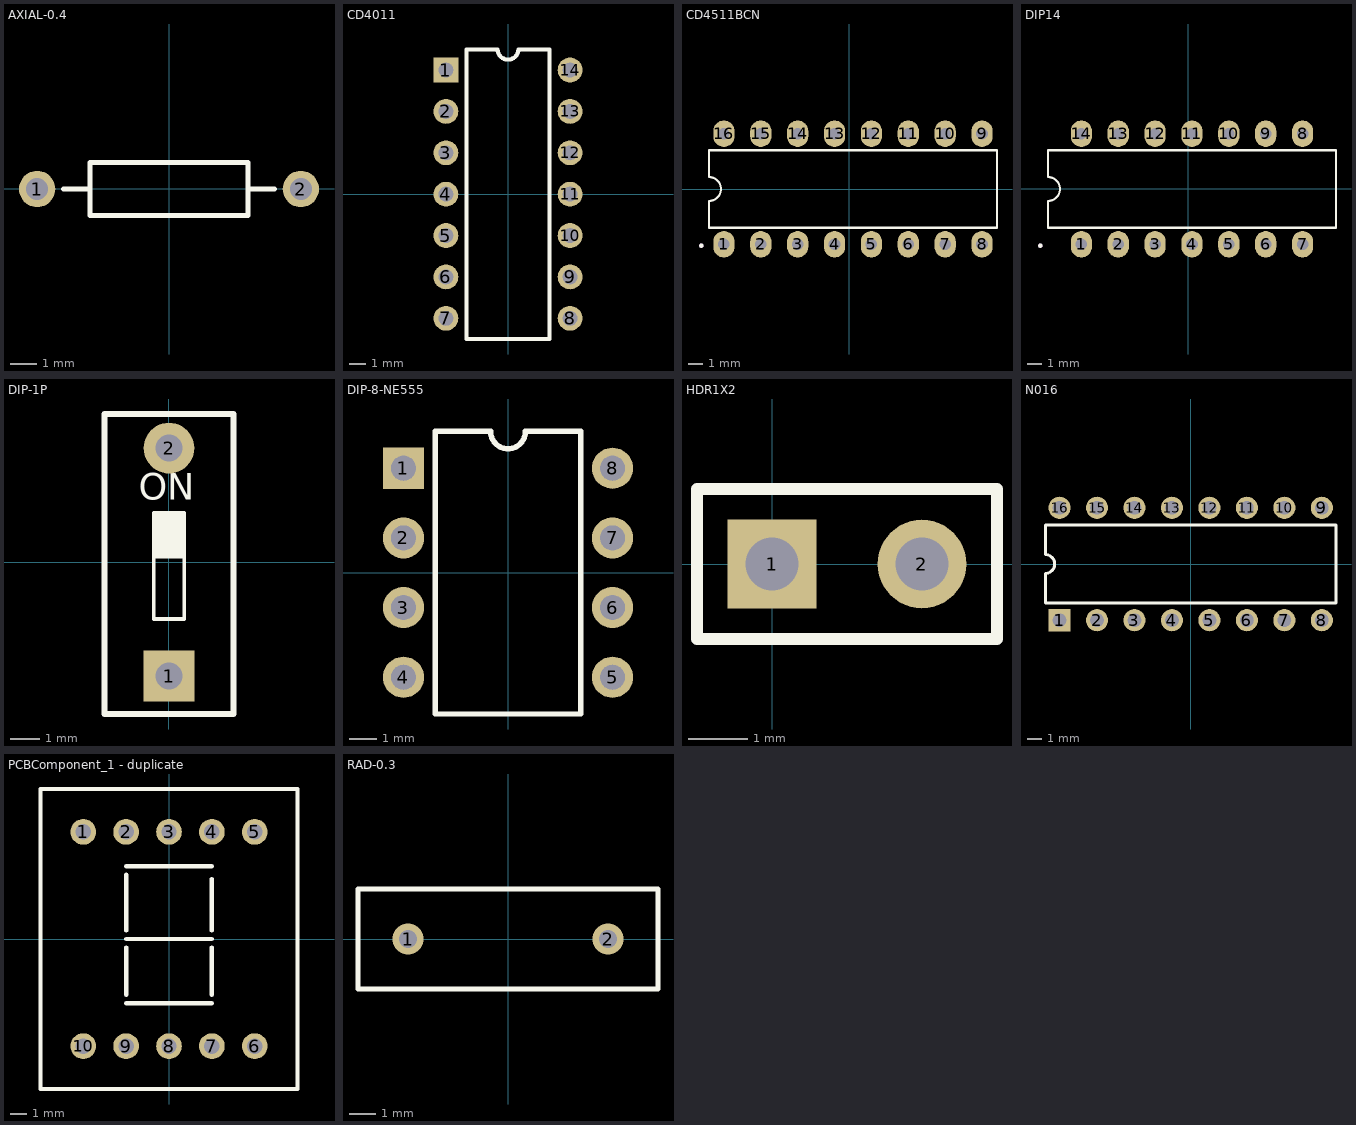
[diagram p0: the footprints below, top view; thin cyan lines are the x and y axes]
# Altium footprint library MISC80628-23.PcbLib: 10 footprints
Each footprint in its own frame and in the unit in brackets; x right, y up, seen from the top. Pads: shape width x height; smd on the part's side, far side on the other; paste and mask are expansions set on the pad; w line width, h text height; cw(c..) or ccw(c..) is an arc to the next point about the centre after c.

## AXIAL-0.4 [mm]
pads (2):
  round 1.4 hole 0.85: 1(-5.08,0) 2(5.08,0)
Top Overlay:
  lines w0.2: -4.064,0 -3.048,0 ; 3.048,0 4.064,0 ; -3.048,-1.016 3.048,-1.016 3.048,1.016 -3.048,1.016 -3.048,-1.016

## CD4011 [mil]
pads (14):
  rect 60x60 hole 35 slot 35.2 at 0 deg paste+0 mask+2: 1(-150,300)
  round 60 hole 35 slot 35.2 at 0 deg paste+0 mask+2: 2(-150,200) 3(-150,100) 4(-150,0) 5(-150,-100) 6(-150,-200) 7(-150,-300) 8(150,-300) 9(150,-200) 10(150,-100) 11(150,0) 12(150,100) 13(150,200) 14(150,300)
Top Overlay:
  lines w10: -100,-350 100,-350 100,350 25,350 cw(c0,350) -25,350 -100,350 -100,-350

## CD4511BCN [mm]
pads (16):
  oval 1.462x1.828 hole 0.8 paste+0 mask+0.051: 1(-8.628,-3.81) 2(-6.088,-3.81) 3(-3.548,-3.81) 4(-1.008,-3.81) 5(1.532,-3.81) 6(4.072,-3.81) 7(6.612,-3.81) 8(9.152,-3.81) 9(9.152,3.81) 10(6.612,3.81) 11(4.072,3.81) 12(1.532,3.81) 13(-1.008,3.81) 14(-3.548,3.81) 15(-6.088,3.81) 16(-8.628,3.81)
Top Overlay:
  circle w0.15: c-10.185,-3.902 r0.075
  lines w0.152: -9.659,-0.825 ccw(c-9.659,0) -9.659,0.825 -9.659,2.668 10.184,2.668 10.184,-2.668 -9.659,-2.668 -9.659,-0.825
Mechanical 15:
  circle w0.15: c-10.185,-3.902 r0.075

## DIP14 [mm]
pads (14):
  oval 1.462x1.827 hole 0.8 paste+0 mask+0.051: 1(-7.358,-3.81) 2(-4.818,-3.81) 3(-2.278,-3.81) 4(0.262,-3.81) 5(2.802,-3.81) 6(5.342,-3.81) 7(7.882,-3.81) 8(7.882,3.81) 9(5.342,3.81) 10(2.802,3.81) 11(0.262,3.81) 12(-2.278,3.81) 13(-4.818,3.81) 14(-7.358,3.81)
Top Overlay:
  circle w0.15: c-10.185,-3.902 r0.075
  lines w0.152: -9.659,0.825 cw(c-9.659,0) -9.659,-0.825 -9.659,-2.668 10.184,-2.668 10.184,2.668 -9.659,2.668 -9.659,0.825
Mechanical 15:
  circle w0.15: c-10.185,-3.902 r0.075

## DIP-1P [mm]
pads (2):
  rect 1.7x1.7 hole 0.9: 1(0,-3.81)
  round 1.7 hole 0.9: 2(0,3.81)
Top Overlay:
  rectangle: -0.508,0.127 0.508,1.651
  lines w0.127: -0.508,-1.905 0.508,-1.905 0.508,1.651 -0.508,1.651 -0.508,-1.905
  lines w0.2: -2.159,-5.08 2.159,-5.08 2.159,4.953 -2.159,4.953 -2.159,-5.08
  text "ON" at -1.016,1.778 h1.52
3D body "DIP-1P.STEP": height 6.65, standoff -3.15, extent -2.068,-4.953 2.032,4.947

## DIP-8-NE555 [mm]
pads (8):
  rect 1.5x1.5 hole 0.9 slot 0.905 at 0 deg paste+0 mask+0.051: 1(-3.81,3.81)
  round 1.5 hole 0.9 slot 0.905 at 0 deg paste+0 mask+0.051: 2(-3.81,1.27) 3(-3.81,-1.27) 4(-3.81,-3.81) 5(3.81,-3.81) 6(3.81,-1.27) 7(3.81,1.27) 8(3.81,3.81)
Top Overlay:
  lines w0.2: -0.635,5.15 -2.65,5.15 -2.65,-5.15 2.65,-5.15 2.65,5.15 0.635,5.15 ; -0.635,5.151 ccw(c0,5.151) 0.635,5.151

## HDR1X2 [mm]
pads (2):
  rect 1.5x1.5 hole 0.9: 1(0,0)
  round 1.5 hole 0.9: 2(2.54,0)
Top Overlay:
  lines w0.2: -1.27,-1.27 -1.27,1.27 3.81,1.27 3.81,-1.27 -1.27,-1.27

## N016 [mm]
pads (16):
  rect 1.5x1.5 hole 0.9 slot 0.905 at 90 deg paste+0 mask+0.051: 1(-8.89,-3.81)
  round 1.5 hole 0.9 slot 0.905 at 90 deg paste+0 mask+0.051: 2(-6.35,-3.81) 3(-3.81,-3.81) 4(-1.27,-3.81) 5(1.27,-3.81) 6(3.81,-3.81) 7(6.35,-3.81) 8(8.89,-3.81) 9(8.89,3.81) 10(6.35,3.81) 11(3.81,3.81) 12(1.27,3.81) 13(-1.27,3.81) 14(-3.81,3.81) 15(-6.35,3.81) 16(-8.89,3.81)
Top Overlay:
  lines w0.2: -9.85,-2.65 -9.85,-0.635 ccw(c-9.85,0) -9.85,0.635 -9.85,2.65 9.85,2.65 9.85,-2.65 -9.85,-2.65

## PCBComponent_1 - duplicate [mil]
pads (10):
  round 60 hole 36 paste+0 mask+2: 1(-200,250) 2(-100,250) 3(0,250) 4(100,250) 5(200,250) 6(200,-250) 7(100,-250) 8(0,-250) 9(-100,-250) 10(-200,-250)
Top Overlay:
  lines w10: -100,-150 100,-150 ; -100,-130 -100,-20 ; -100,0 100,0 ; -100,20 -100,150 ; -100,170 100,170 ; 100,-130 100,-20 ; 100,20 100,140 ; -300,-350 -300,350 300,350 300,-350 -300,-350

## RAD-0.3 [mm]
pads (2):
  round 1.2 hole 0.7: 1(-3.81,0) 2(3.81,0)
Top Overlay:
  lines w0.2: -5.715,-1.905 -5.715,1.905 5.715,1.905 5.715,-1.905 -5.715,-1.905